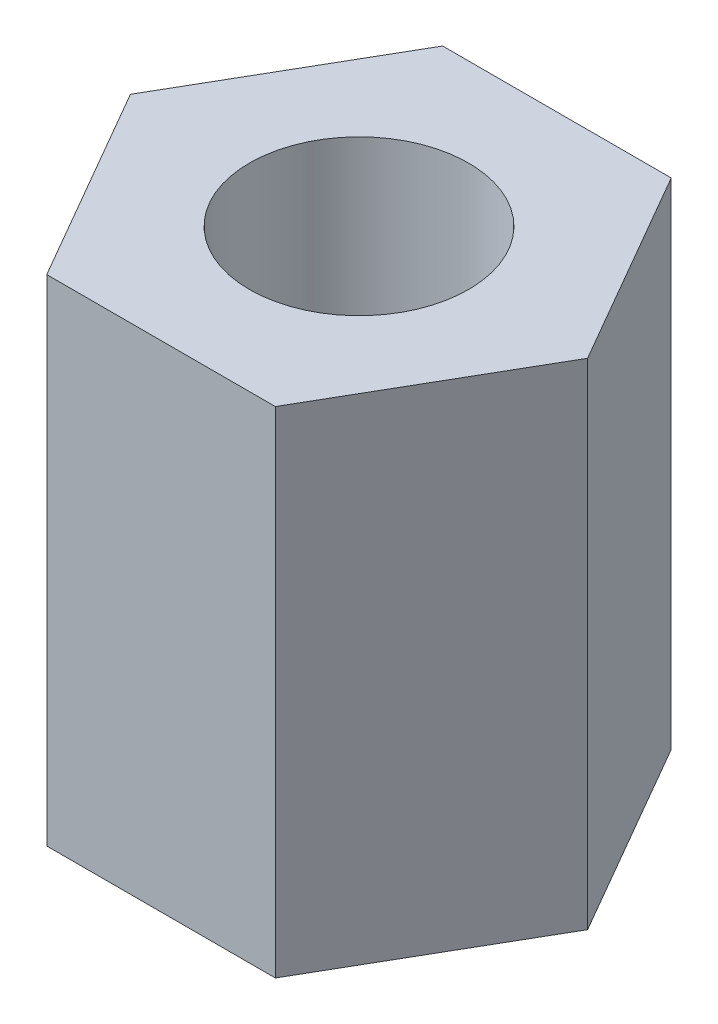
from build123d import *

# Parameters (mm, degrees)
SKETCH_1_R      = 1.55
EXTRUDE_1_DEPTH = 7


with BuildPart() as part:
    # 草图1 → 凸台-拉伸1 (new body)
    with BuildSketch(Plane(origin=(0, 0, 0), x_dir=(1, 0, 0), z_dir=(0, 1, 0))):
        Polygon((1.616580754, -2.8), (3.233161507, 0), (1.616580754, 2.8), (-1.616580754, 2.8), (-3.233161507, 0), (-1.616580754, -2.8), align=None)
        with Locations(Location((0, 0, 0), (0, 0, 270))):
            Circle(SKETCH_1_R, mode=Mode.SUBTRACT)
    extrude(amount=EXTRUDE_1_DEPTH)


solid = part.part
